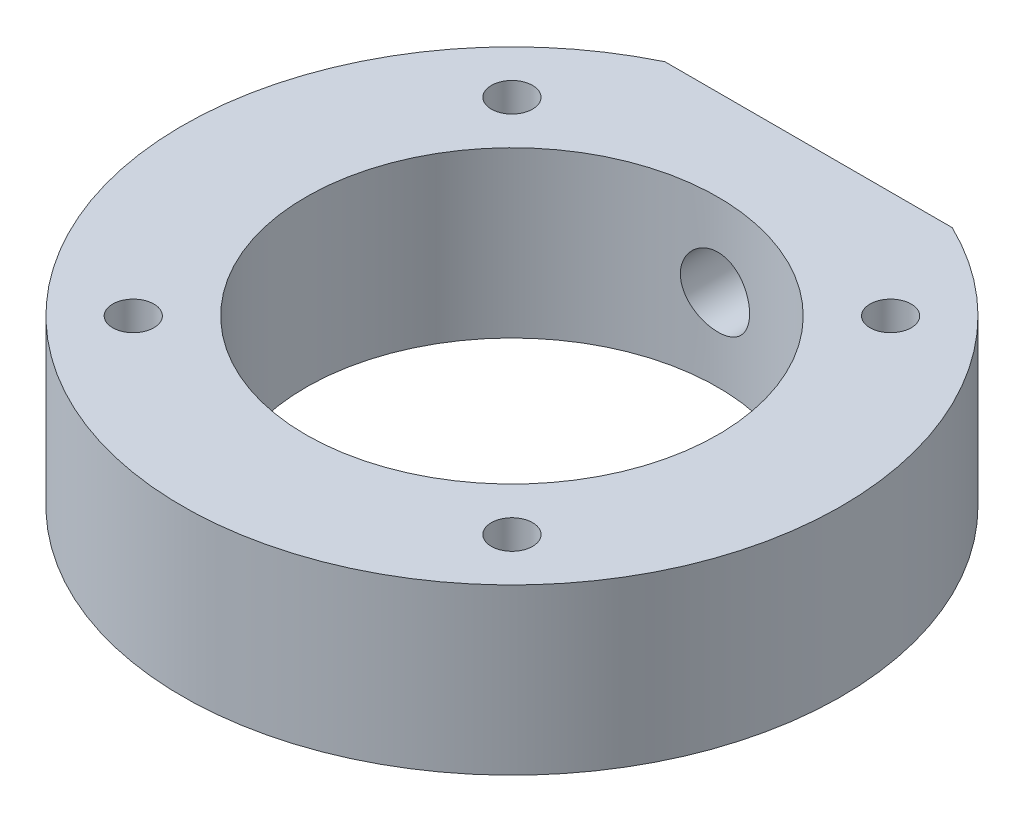
from build123d import *

# Parameters (mm, degrees)
SKETCH1_R              = 20
SKETCH1_R_2            = 12.5
BOSS_EXTRUDE1_DEPTH    = 10
CUT_EXTRUDE1_DEPTH     = 31
M5_TAPPED_HOLE1_REACH  = 46.091
M5_TAPPED_HOLE1_BORE_R = 2.1
M3_TAPPED_HOLE1_D      = 2.5


with BuildPart() as part:
    # Sketch1 → Boss-Extrude1 (new body)
    with BuildSketch(Plane(origin=(0, 0, 0), x_dir=(1, 0, 0), z_dir=(0, 1, 0))):
        with Locations(Location((0, 0, 0), (0, 0, 270))):
            Circle(SKETCH1_R)
        with Locations(Location((0, 0, 0), (0, 0, 270))):
            Circle(SKETCH1_R_2, mode=Mode.SUBTRACT)
    extrude(amount=BOSS_EXTRUDE1_DEPTH)

    # Sketch2 → Cut-Extrude1 (cut, through all)
    with BuildSketch(Plane(origin=(0, 10, 0), x_dir=(1, 0, 0), z_dir=(0, 1, 0))):
        with BuildLine():
            Line((8.717797887, 18), (-8.717797887, 18))
            ThreePointArc((-8.717797887, 18), (0, 20), (8.717797887, 18))
        make_face()
    extrude(amount=-CUT_EXTRUDE1_DEPTH, mode=Mode.SUBTRACT)

    # M5 Tapped Hole1 bore → M5 Tapped Hole1 (cut, up to next)
    with BuildSketch(Plane(origin=(0, 0, -18), x_dir=(-1, 0, 0), z_dir=(0, 0, -1)), mode=Mode.PRIVATE) as m5_tapped_hole1_sk1:
        with Locations((0, 5)):
            Circle(M5_TAPPED_HOLE1_BORE_R)
    m5_tapped_hole1_tool1 = extrude(m5_tapped_hole1_sk1.sketch, amount=-M5_TAPPED_HOLE1_REACH, mode=Mode.PRIVATE) & part.part
    add(m5_tapped_hole1_tool1.solids().sort_by_distance((0, 5, -18))[0], mode=Mode.SUBTRACT)

    # M3 Tapped Hole1 (through all)
    with Locations(Plane(origin=(0, 0, 0), x_dir=(-1, 0, 0), z_dir=(0, -1, 0))):
        with Locations((-11.490485194, 11.490485194), (11.490485194, 11.490485194), (-11.490485194, -11.490485194), (11.490485194, -11.490485194)):
            Hole(M3_TAPPED_HOLE1_D / 2)


solid = part.part
